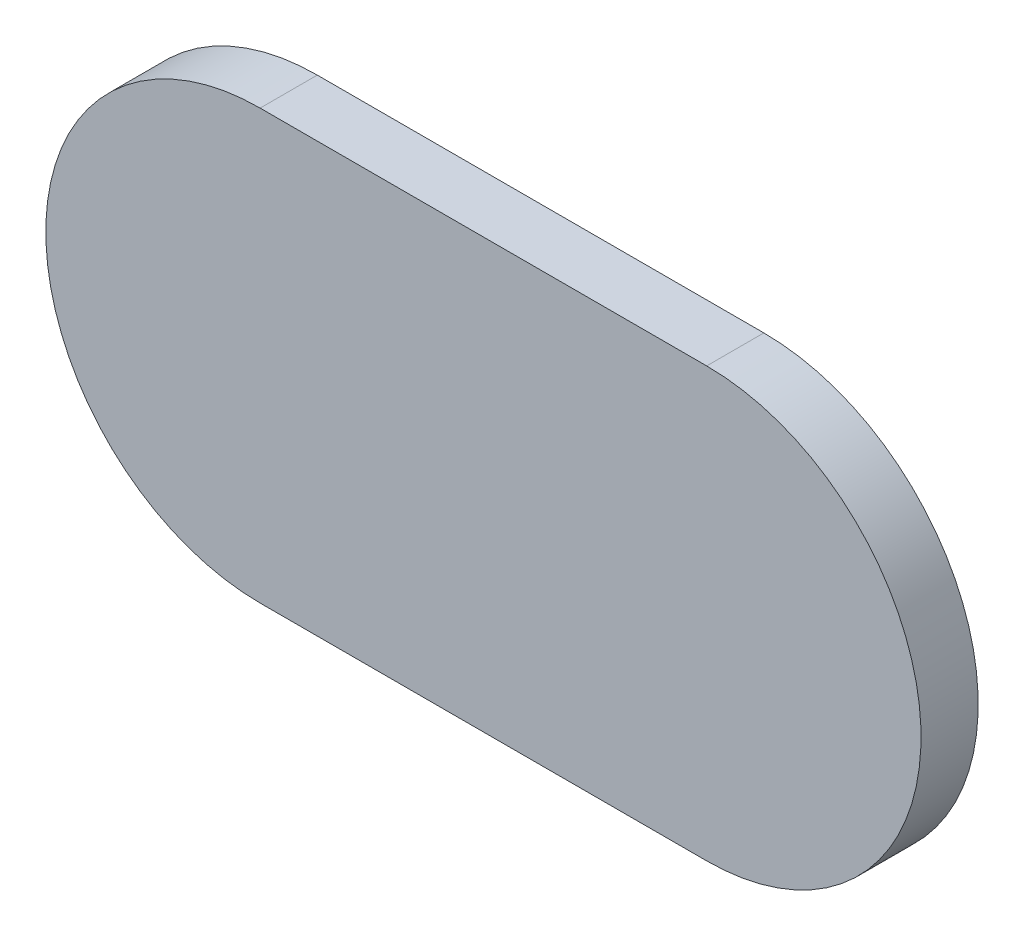
SolidWorks part; units mm, degrees
material "Q345 "
ref_plane "前视基准面" through (0, 0, 0) normal (0, 0, 1) x (1, 0, 0)
ref_plane "上视基准面" through (0, 0, 0) normal (0, 1, 0) x (1, 0, 0)
ref_plane "右视基准面" through (0, 0, 0) normal (1, 0, 0) x (0, 0, -1)
sketch "草图1" plane through (0, 0, 0) normal (0, 0, 1) x (1, 0, 0)
  line L0 (-62.5, 0) -> (62.5, 0) construction
  line L1 (-62.5, 60) -> (62.5, 60)
  line L2 (-62.5, -60) -> (62.5, -60)
  arc A0 (-62.5, 60) -> (-62.5, -60) centre (-62.5, 0) ccw
  arc A1 (62.5, -60) -> (62.5, 60) centre (62.5, 0) ccw
  point P2 (0, 0)
  dimension "D1" = 60
  dimension "D2" = 125
extrude "凸台-拉伸1" add sketch "草图1" along normal blind 16
